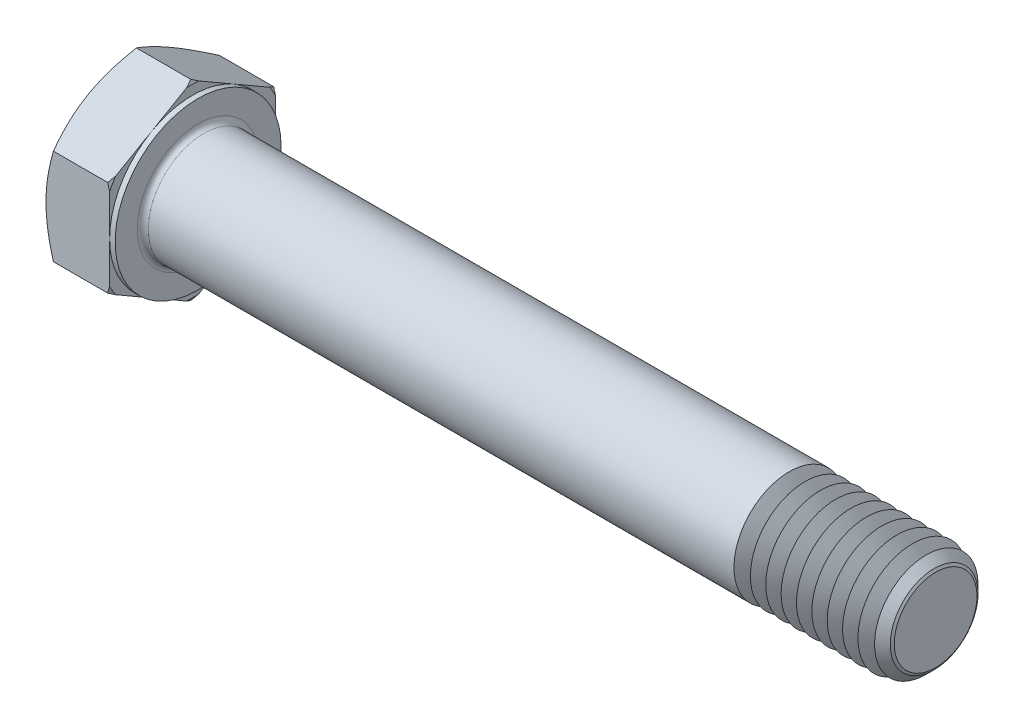
SolidWorks part; units mm, degrees
extrude "基体-拉伸" add sketch "草图1" along normal blind 7.5
sketch "草图1" plane through (0, 0, 0) normal (1, 0, 0) x (0, 0, -1)
  line L0 (9, 5.1962) -> (9, -5.1962)
  line L1 (-9, 5.1962) -> (-9, -5.1962)
  line L2 (9, -5.1962) -> (0, -10.3923)
  line L3 (0, -10.3923) -> (-9, -5.1962)
  line L4 (9, 5.1962) -> (0, 10.3923)
  line L5 (0, 10.3923) -> (-9, 5.1962)
revolve "切除-旋转1" cut sketch "草图3" angle 360 about L6
sketch "草图3" plane through (0, 0, 0) normal (0, 0, 1) x (1, 0, 0)
  line L0 (0, 9) -> (3.6906, 15.3923)
  line L1 (0, 10.3923) -> (0, 5.1962) construction
  line L2 (3.6906, 15.3923) -> (3.6906, 20.3923)
  line L3 (3.6906, 20.3923) -> (-10, 20.3923)
  line L4 (-10, 20.3923) -> (-10, 9)
  line L5 (-10, 9) -> (0, 9)
  line L6 (0, 0) -> (99.06, 0) construction
  line L7 (7.5, 10.3923) -> (0, 10.3923) construction
material "5.6级"
ref_plane "前视" through (0, 0, 0) normal (0, 0, 1) x (1, 0, 0)
ref_plane "上视" through (0, 0, 0) normal (0, 1, 0) x (1, 0, 0)
ref_plane "右视" through (0, 0, 0) normal (1, 0, 0) x (0, 0, -1)
sketch "草图2" plane through (0, 0, 0) normal (0, 0, 1) x (1, 0, 0)
  line L0 (0, 5.1962) -> (0, -5.1962) construction
  line L1 (0, 0) -> (87.5, 0)
  line L2 (0, 0) -> (0, 6)
  line L3 (0, 6) -> (7.7917, 6)
  line L4 (87.5, 0) -> (87.5, 4.4845)
  line L5 (7.5, 10.3923) -> (7.5, 5.1962) construction
  line L7 (0, 0) -> (96.52, 0) construction
  line L8 (87.5, -4.4845) -> (7.7917, -6) construction
  line L9 (0, -6) -> (7.7917, -6) construction
  line L10 (9.25, 15.24) -> (9.25, -1.27) construction
  line L11 (72.5, 15.24) -> (72.5, -1.27) construction
  line L12 (7.5, 5.1962) -> (7.5, -5.1962) construction
  line L13 (7.7917, 6) -> (87.5, 6)
  line L14 (87.5, 6) -> (87.5, 4.4845)
revolve "凸台-旋转1" add sketch "草图2" angle 360 about L7
cosmetic thread "螺旋线1" parameters "Thread_length"=15, "Thread_minor"=8.969
sketch "草图5" plane through (0, 0, 0) normal (0, 0, 1) x (1, 0, 0)
  line L0 (7.5, 9) -> (3.8094, 15.3923)
  line L1 (7.5, 10.3923) -> (7.5, 5.1962) construction
  line L2 (3.8094, 15.3923) -> (3.8094, 20.3923)
  line L3 (3.8094, 20.3923) -> (13.8094, 20.3923)
  line L4 (13.8094, 20.3923) -> (13.8094, 9)
  line L5 (13.8094, 9) -> (7.5, 9)
  line L7 (7.5, 10.3923) -> (0.8038, 10.3923) construction
  line L8 (0, 0) -> (99.06, 0) construction
  line L9 (0, 0) -> (99.06, 0) construction
revolve "切除-旋转2" cut sketch "草图5" angle 360 about L8
sketch "草图4" plane through (0, 0, 0) normal (0, 0, 1) x (1, 0, 0)
  line L1 (7.5, 10.3923) -> (7.5, 5.1962) construction
  line L2 (7.5, 9) -> (6.9, 9)
  line L3 (7.5, 9) -> (7.5, 20.3923)
  line L4 (7.5, 20.3923) -> (6.9, 20.3923)
  line L5 (0, 0) -> (95.25, 0) construction
  line L6 (0, 0) -> (96.52, 0) construction
  line L7 (6.9, 9) -> (6.9, 20.3923)
  line L8 (6.6962, 10.3923) -> (0.8038, 10.3923) construction
revolve "切除-旋转3" cut sketch "草图4" angle 360 about L5
chamfer "倒角" distance 1.4 angle 45 1 edges at (87.5, 0, 6)
fillet "圆角" radius 0.6 1 edges at (7.5, 0, -6)
sketch "草图6" plane through (0, 0, 0) normal (0, 0, 1) x (1, 0, 0)
  line L0 (72.5, -4.4845) -> (71.625, -6)
  line L1 (72.5, -4.4845) -> (73.375, -6)
  line L2 (73.375, -6) -> (73.375, -7.5)
  line L3 (-3.175, 0) -> (5.1513, 0) construction
  line L5 (73.375, -7.5) -> (71.625, -7.5)
  line L6 (71.625, -7.5) -> (71.625, -6)
revolve "切除-旋转4" cut sketch "草图6" angle 360 about L3
pattern_linear "阵列(线性)1" count 10 spacing 1.6667 along (1, 0, 0) of "切除-旋转4"
equation "\"D3@草图1\" = \"s@草图1\" / 2"
equation "\"D4@草图1\" = \"D3@草图1\""
equation "\"D5@草图1\" = \"D4@草图1\""
equation "\"Thread_minor@螺旋线1\" = \"Minor_dia@草图2\""
equation "\"D1@草图3\" = \"s@草图1\" / 2"
equation "\"D1@草图5\" = \"s@草图1\" / 2"
equation "\"Head_ch_ang@草图5\" = \"Head_ch_ang@草图3\""
equation "\"D1@草图4\" = \"s@草图1\""
equation "\"Thread_length@螺旋线1\" = ((sgn( (\"l@草图2\" - \"p@草图2\" ) - \"h@草图2\" )-1)*( (\"l@草图2\" - \"p@草图2\" ) - \"h@草图2\" ))/-2+ \"h@草图2\""
equation "\"Thread_minor@草图6\" = \"Minor_dia@草图2\""
equation "\"Diameter@草图6\" = \"m@草图2\""
equation "\"Overcut@草图6\" = \"m@草图2\" * 1.25"
equation "\"Start@草图6\" = \"k@基体-拉伸\" + \"l@草图2\" - \"Thread_length@螺旋线1\"  '---Non-countersunk---"
equation "\"Num_threads@阵列(线性)1\" = int( \"Thread_length@螺旋线1\" / \"p@草图2\" + 0.999 )  + 1"
equation "\"Advance@阵列(线性)1\" = \"Thread_length@螺旋线1\" /  (\"Num_threads@阵列(线性)1\" - 1) 'relax it"
equation "\"Num_threads@阵列(线性)1\" = \"Num_threads@阵列(线性)1\" - sgn( \"Num_threads@阵列(线性)1\" - 1) '---chamfered tips only---"
equation "\"Minor_dia@草图2\" = \"m@草图2\"-\"p@草图2\" * 1.732"
equation "\"D1@倒角\" = \"p@草图2\"*0.8"
